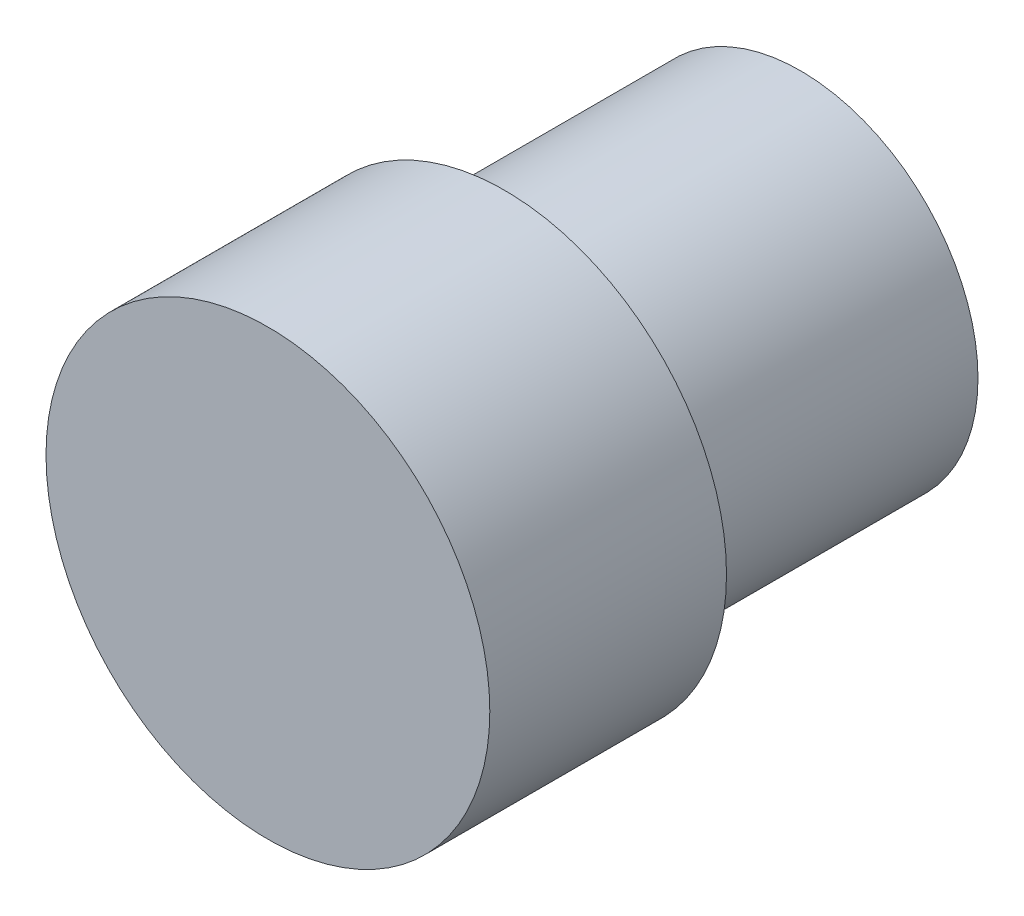
from build123d import *

# Parameters (mm, degrees)
SKETCH_1_R      = 6
EXTRUDE_1_DEPTH = 10
SKETCH_2_R      = 7.5
EXTRUDE_2_DEPTH = 8


with BuildPart() as part:
    # 草图1 → 凸台-拉伸1 (new body)
    with BuildSketch(Plane.XY):
        Circle(SKETCH_1_R)
    extrude(amount=-EXTRUDE_1_DEPTH)

    # 草图2 → 凸台-拉伸2 (add)
    with BuildSketch(Plane.XY):
        Circle(SKETCH_2_R)
    extrude(amount=EXTRUDE_2_DEPTH)


solid = part.part
